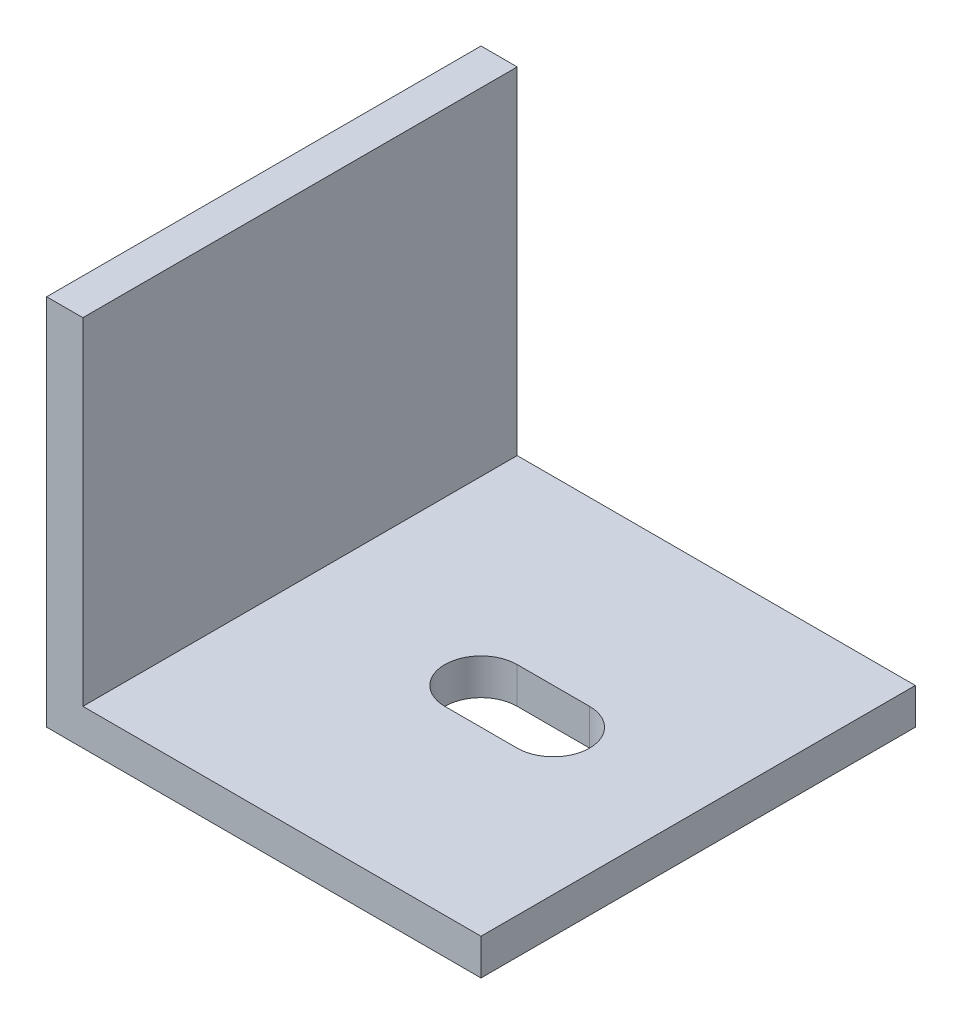
from build123d import *

# Parameters (mm, degrees)
EXTRUDE_THIN1_DEPTH = 60
CUT_EXTRUDE1_DEPTH  = 164.245214325


with BuildPart() as part:
    # Sketch1 → Extrude-Thin1 (new, symmetric)
    with BuildSketch(Plane.XY):
        Polygon((120, 0), (0, 0), (0, 103), (10, 103), (10, 10), (120, 10), align=None)
    extrude(amount=EXTRUDE_THIN1_DEPTH, both=True)

    # Sketch2 → Cut-Extrude1 (cut, through all)
    with BuildSketch(Plane(origin=(0, 10, 0), x_dir=(1, 0, 0), z_dir=(0, 1, 0))):
        with BuildLine():
            Line((60, 10), (80, 10))
            ThreePointArc((80, 10), (90, 0), (80, -10))
            Line((80, -10), (60, -10))
            ThreePointArc((60, -10), (50, 0), (60, 10))
        make_face()
    extrude(amount=-CUT_EXTRUDE1_DEPTH, mode=Mode.SUBTRACT)


solid = part.part
